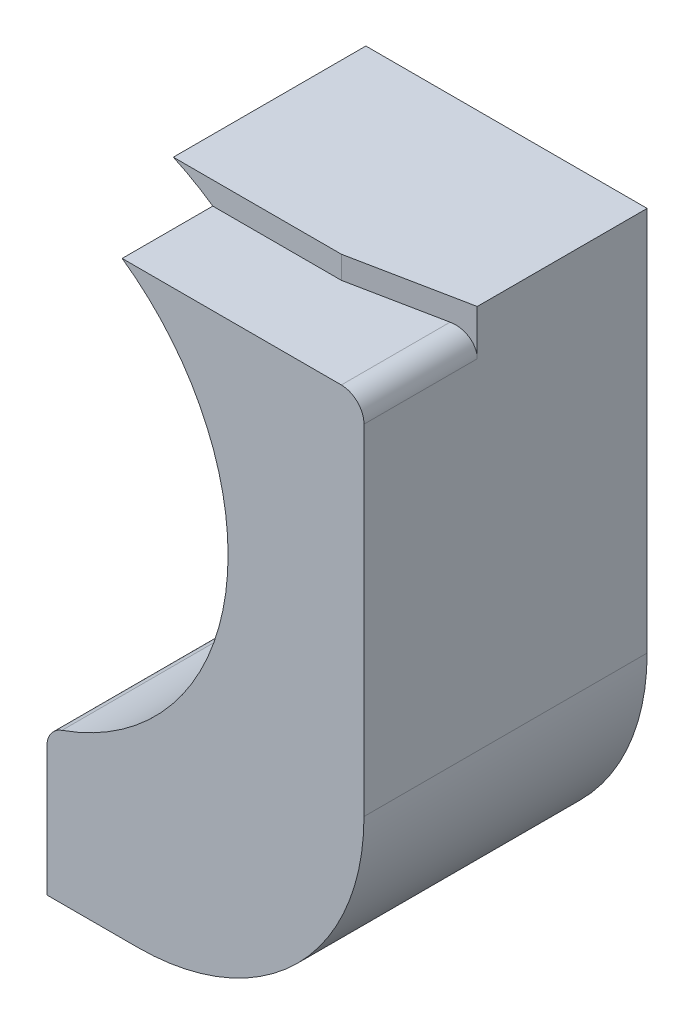
SolidWorks part; units mm, degrees
ref_plane "前视基准面" through (0, 0, 0) normal (0, 0, 1) x (1, 0, 0)
ref_plane "上视基准面" through (0, 0, 0) normal (0, 1, 0) x (1, 0, 0)
ref_plane "右视基准面" through (0, 0, 0) normal (1, 0, 0) x (0, 0, -1)
sketch "草图1" plane through (0, 0, 0) normal (0, 0, 1) x (1, 0, 0)
  line L0 (-7, -7.083) -> (-7, -13.5)
  line L1 (7, 13.5) -> (-5.4174, 13.5)
  line L2 (7, 13.5) -> (7, -13.5)
  line L3 (7, -13.5) -> (-7, -13.5)
  line L5 (7, 13.5) -> (-7, -13.5) construction
  line L6 (7, -13.5) -> (-7, 13.5) construction
  arc A0 (-7, -7.083) -> (-5.4174, 13.5) centre (-10, 3.5) ccw
  point P0 (0, 0)
  dimension "D2" = 11
  dimension "D5" = 17
  dimension "D1" = 27
  dimension "D3" = 14
  dimension "D4" = 10
extrude "凸台-拉伸1" add sketch "草图1" along normal blind 12.5
sketch "草图2" plane through (0, 13.5, 0) normal (0, 1, 0) x (1, 0, 0)
  line L0 (-5.4174, -12.5) -> (-5.4174, -8.5)
  line L1 (-5.4174, -12.5) -> (-5.4174, 0) construction
  line L2 (-5.4174, -8.5) -> (2, -8.5)
  line L3 (2, -8.5) -> (7, -7.5)
  line L4 (7, -12.5) -> (7, 0) construction
  line L5 (7, -7.5) -> (7, -12.5)
  line L6 (7, -12.5) -> (-5.4174, -12.5)
  dimension "D1" = 4
  dimension "D2" = 5
  dimension "D3" = 5
extrude "切除-拉伸1" cut sketch "草图2" against normal blind 1
fillet "圆角1" radius 10 1 edges at (7, -13.5, 6.25)
fillet "圆角2" radius 1 1 edges at (7, 12.5, 10)
hole_wizard "M2 螺纹孔1" positions "草图4" profile "草图3" tap size "M2" standard "Iso"
sketch "草图4" plane through (0, 0, 0) normal (0, 0, -1) x (-1, 0, 0)
  point P0 (-4, 2.5)
  point P3 (-4, 10.5)
sketch "草图3" plane through (4, 2.5, 0) normal (1, 0, 0) x (0, 1, 0)
  line L0 (0, 0) -> (0, 5.6807)
  line L1 (0, 5.6807) -> (0.8, 5.2)
  line L2 (0.8, 5.2) -> (0.8, 0)
  line L5 (0.8, 0) -> (0, 0)
  line L10 (0, 5.6807) -> (-0.8, 5.2) construction
  line L11 (0, -6.35) -> (0, 107.95) construction
  dimension "螺纹孔钻头直径" = 1.6
  dimension "螺纹孔钻头深度" = 5.2
  dimension "导头角度" = 118
cosmetic thread "孔螺蚊线1" parameters "D1"=4, "D2"=2
cosmetic thread "孔螺蚊线2" parameters "D1"=4, "D2"=2
fillet "圆角4" radius 1 1 edges at (-7, -7.083, 6.25)
